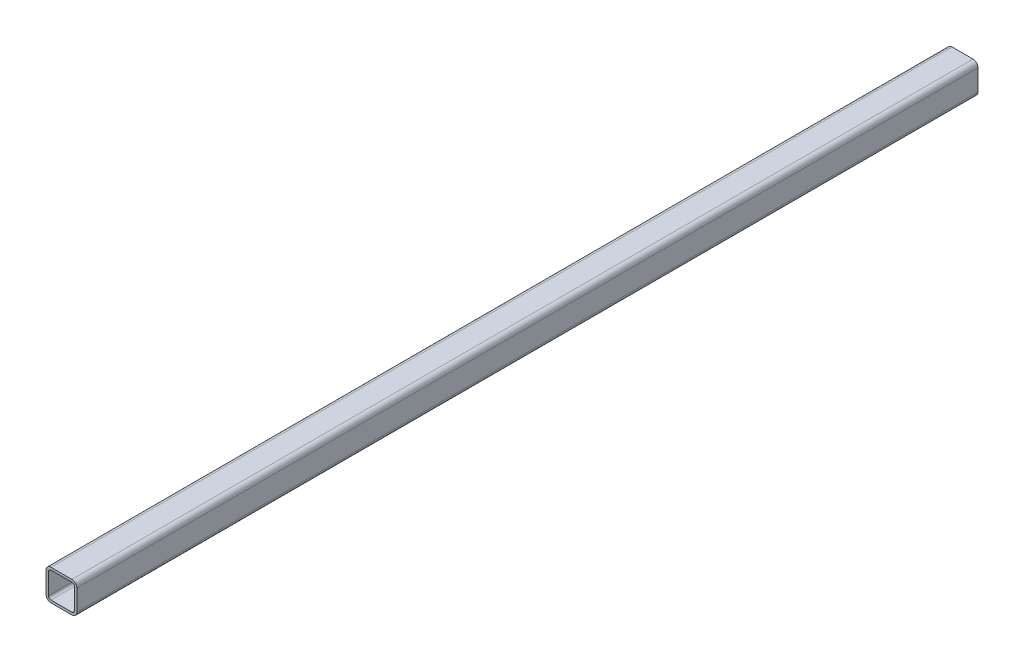
SolidWorks part; units mm, degrees
material "Q235"
ref_plane "Plane1" through (0, 0, 0) normal (0, 0, 1) x (1, 0, 0)
ref_plane "Plane2" through (0, 0, 0) normal (0, 1, 0) x (1, 0, 0)
ref_plane "Plane3" through (0, 0, 0) normal (1, 0, 0) x (0, 0, -1)
sketch "Sketch1" plane through (0, 0, 0) normal (0, 0, 1) x (1, 0, 0)
  line L0 (-8.5, -10.5) -> (8.5, -10.5)
  line L1 (-10.5, -8.5) -> (-10.5, 8.5)
  line L2 (8.5, 10.5) -> (-8.5, 10.5)
  line L3 (10.5, 8.5) -> (10.5, -8.5)
  line L4 (-8.5, -12.5) -> (8.5, -12.5)
  line L5 (-12.5, -8.5) -> (-12.5, 8.5)
  line L6 (8.5, 12.5) -> (-8.5, 12.5)
  line L7 (12.5, 8.5) -> (12.5, -8.5)
  arc A0 (12.5, 8.5) -> (8.5, 12.5) centre (8.5, 8.5) ccw
  arc A1 (8.5, -12.5) -> (12.5, -8.5) centre (8.5, -8.5) ccw
  arc A2 (-12.5, -8.5) -> (-8.5, -12.5) centre (-8.5, -8.5) ccw
  arc A3 (-8.5, 12.5) -> (-12.5, 8.5) centre (-8.5, 8.5) ccw
  arc A4 (-8.5, 10.5) -> (-10.5, 8.5) centre (-8.5, 8.5) ccw
  arc A5 (10.5, 8.5) -> (8.5, 10.5) centre (8.5, 8.5) ccw
  arc A6 (8.5, -10.5) -> (10.5, -8.5) centre (8.5, -8.5) ccw
  arc A7 (-10.5, -8.5) -> (-8.5, -10.5) centre (-8.5, -8.5) ccw
  point P0 (0, 12.5)
  point P1 (12.5, 0)
  point P2 (0, -12.5)
  point P3 (-12.5, 0)
  point P4 (-12.5, 12.5)
  point P5 (12.5, 12.5)
  point P6 (12.5, -12.5)
  point P7 (-12.5, -12.5)
  point P8 (0, 0)
extrude "Boss-Extrude1" add sketch "Sketch1" along normal blind 730
